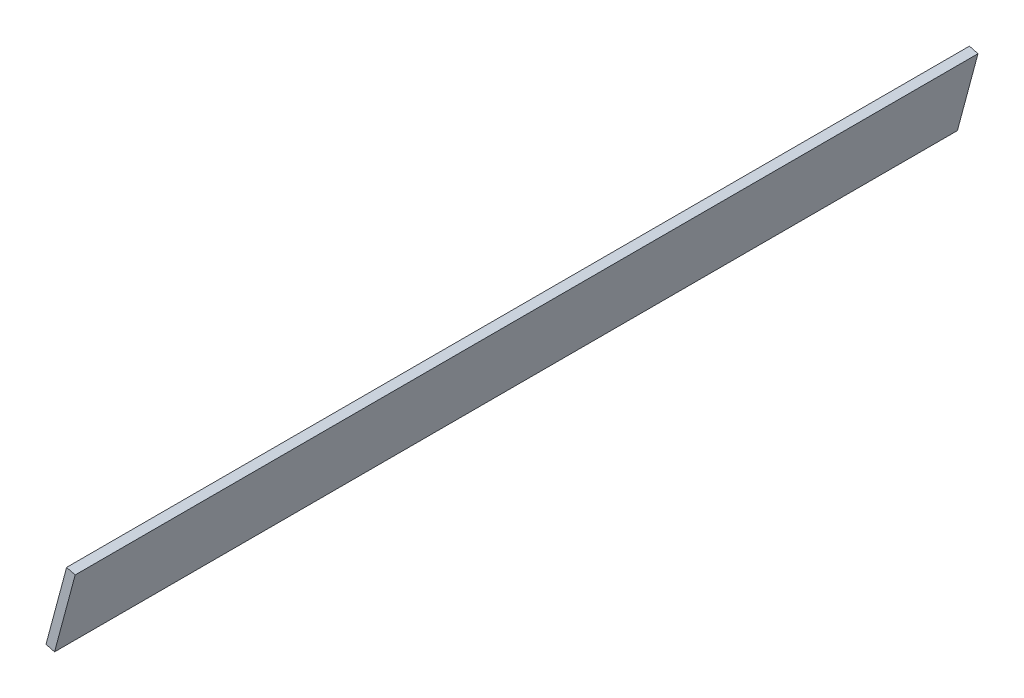
from build123d import *

# Parameters (mm, degrees)
SKETCH_1_W      = 18
SKETCH_1_H      = 204
EXTRUDE_1_DEPTH = 2


with BuildPart() as part:
    # 草图1 → 凸台-拉伸1 (new body)
    with BuildSketch(Plane(origin=(2654.71278719, -711.328147464, 0), x_dir=(-0.25881904510251985, -0.9659258262890685, 0), z_dir=(-0.9659258262890685, 0.25881904510251985, 0))):
        with Locations((-2148.780959522, 190.144615796)):
            Rectangle(SKETCH_1_W, SKETCH_1_H)
    extrude(amount=-EXTRUDE_1_DEPTH)


solid = part.part
